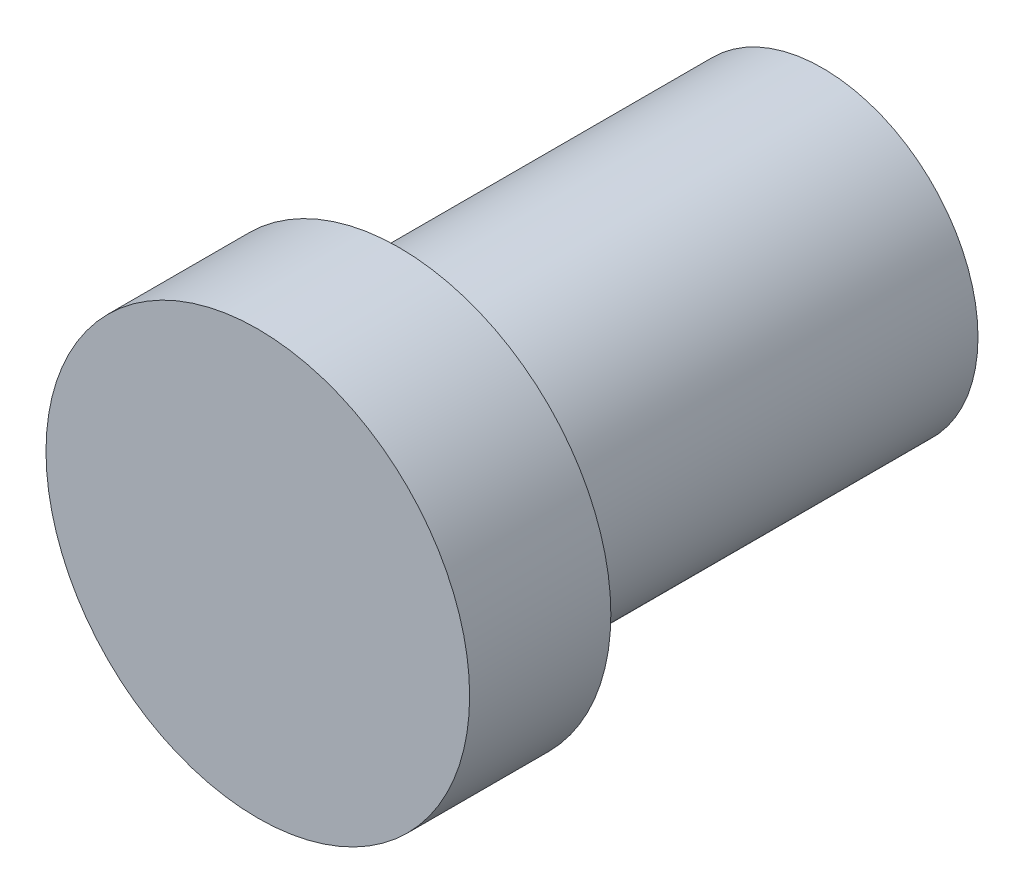
SolidWorks part; units mm, degrees
ref_plane "前视基准面" through (0, 0, 0) normal (0, 0, 1) x (1, 0, 0)
ref_plane "上视基准面" through (0, 0, 0) normal (0, 1, 0) x (1, 0, 0)
ref_plane "右视基准面" through (0, 0, 0) normal (1, 0, 0) x (0, 0, -1)
other "Configuration Table"
sketch "草图1" plane through (0, 0, 0) normal (0, 0, 1) x (1, 0, 0)
  circle A0 centre (0, 0) radius 2.2
  point P0 (0, 0)
  dimension "D1" = 4.4
extrude "凸台-拉伸1" add sketch "草图1" against normal blind 6
sketch "草图2" plane through (0, 0, 0) normal (0, 0, 1) x (1, 0, 0)
  circle A0 centre (0, 0) radius 3
  point P0 (0, 0)
  dimension "D1" = 6
extrude "凸台-拉伸2" add sketch "草图2" along normal blind 2
